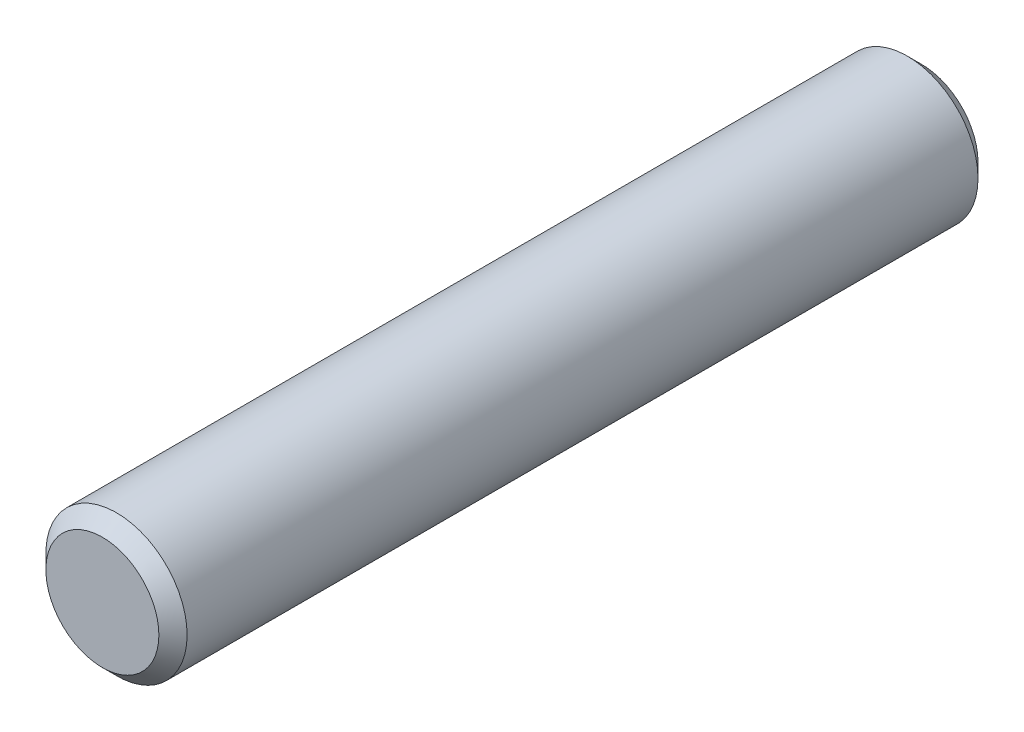
from build123d import *

# Parameters (mm, degrees)
SKETCH1_R           = 0.5
BOSS_EXTRUDE1_DEPTH = 2.9
CHAMFER1_SIZE       = 0.1


with BuildPart() as part:
    # Sketch1 → Boss-Extrude1 (new, symmetric)
    with BuildSketch(Plane.XY):
        Circle(SKETCH1_R)
    extrude(amount=BOSS_EXTRUDE1_DEPTH, both=True)

    # Chamfer1
    chamfer1_edges = [part.edges().sort_by_distance(p)[0] for p in [
        (-0.5, 0, -2.9),
        (-0.5, 0, 2.9),
    ]]
    chamfer(chamfer1_edges, length=CHAMFER1_SIZE)


solid = part.part
